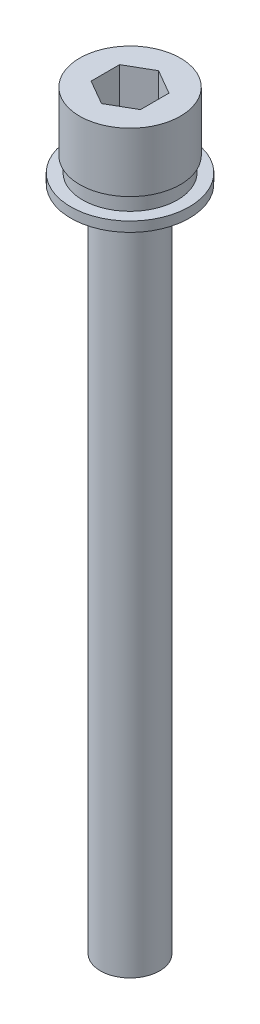
SolidWorks part; units mm, degrees
ref_plane "Front Plane" through (0, 0, 0) normal (0, 0, 1) x (1, 0, 0)
ref_plane "Top Plane" through (0, 0, 0) normal (0, 1, 0) x (1, 0, 0)
ref_plane "Right Plane" through (0, 0, 0) normal (1, 0, 0) x (0, 0, -1)
sketch "Sketch 1" plane through (0, 0, 0) normal (0, 0, 1) x (1, 0, 0)
  line L0 (0, 11.322) -> (0, -25.8305) construction
  line L1 (-9.8983, 0) -> (13.1525, 0) construction
  line L2 (0, 6) -> (-5.1, 6)
  line L3 (-5.1, 6) -> (-5.1, 0)
  line L4 (-5.1, 0) -> (-3, 0)
  line L5 (-3, 0) -> (-3, -70)
  line L6 (-3, -70) -> (0, -70)
  line L7 (0, -70) -> (0, 6)
  dimension "D1" = 6
  dimension "D2" = 70
  dimension "D3" = 6
  dimension "D4" = 10.2
revolve "Revolve 1" add sketch "Sketch 1" angle 360 about L0
sketch "Sketch 2" plane through (0, 6, 0) normal (0, 1, 0) x (1, 0, 0)
  line L1 (0, 2.8868) -> (-2.5, 1.4434)
  line L2 (-2.5, 1.4434) -> (-2.5, -1.4434)
  line L3 (-2.5, -1.4434) -> (0, -2.8868)
  line L4 (0, -2.8868) -> (2.5, -1.4434)
  line L5 (2.5, -1.4434) -> (2.5, 1.4434)
  line L6 (2.5, 1.4434) -> (0, 2.8868)
  circle A0 centre (0, 0) radius 2.5 construction
  dimension "D1" = 5
extrude "Cut-Extrude 1" cut sketch "Sketch 2" against normal blind 5
sketch "Sketch 3" plane through (0, 0, 0) normal (0, -1, 0) x (1, 0, 0)
  circle A0 centre (0, 0) radius 3
  circle A1 centre (0, 0) radius 4.8
  dimension "D1" = 1.8
  dimension "D2" = 6
extrude "Boss-Extrude 1" add sketch "Sketch 3" along normal blind 1.5 separate body
sketch "Sketch 4" plane through (0, -1.5, 0) normal (0, -1, 0) x (1, 0, 0)
  circle A0 centre (0, 0) radius 6
  circle A1 centre (0, 0) radius 3
  dimension "D1" = 6
  dimension "D2" = 12
extrude "Boss-Extrude 2" add sketch "Sketch 4" along normal blind 1 separate body
